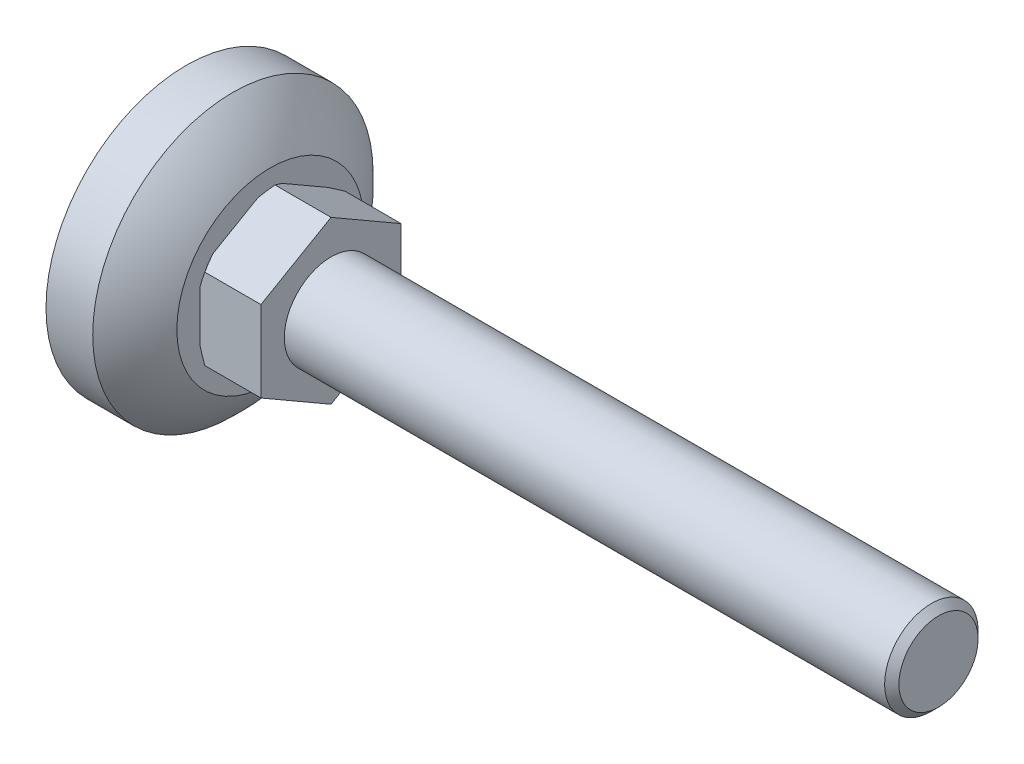
from build123d import *

# Parameters (mm, degrees)
SKETCH2_R          = 19.5
CUT_EXTRUDE1_DEPTH = 13


with BuildPart() as part:
    # Sketch1 → Revolve1 (revolve)
    with BuildSketch(Plane.XY, mode=Mode.PRIVATE) as revolve1_sk:
        with BuildLine():
            Line((0, 0), (0, 30))
            Line((0, 30), (10, 30))
            ThreePointArc((10, 30), (14.390434405, 25.312347524), (18, 20))
            Line((18, 20), (18, 16))
            Line((18, 16), (19.5, 18))
            Line((19.5, 18), (31, 18))
            Line((31, 18), (31, 10))
            Line((31, 10), (159.4665, 10))
            Line((159.4665, 10), (161, 8.4665))
            Line((161, 8.4665), (161, 0))
            Line((161, 0), (0, 0))
        make_face()
    revolve(revolve1_sk.sketch.rotate(Axis((161, 0, 0), (-1, 0, 0)), 270), axis=Axis((161, 0, 0), (-1, 0, 0)))

    # Sketch2 → Cut-Extrude1 (cut)
    with BuildSketch(Plane(origin=(31, 0, 0), x_dir=(0, 0, -1), z_dir=(1, 0, 0))):
        Circle(SKETCH2_R)
        Polygon((-15, 8.660254038), (-15, -8.660254038), (0, -17.320508076), (15, -8.660254038), (15, 8.660254038), (0, 17.320508076), align=None, mode=Mode.SUBTRACT)
    extrude(amount=-CUT_EXTRUDE1_DEPTH, mode=Mode.SUBTRACT)


solid = part.part
